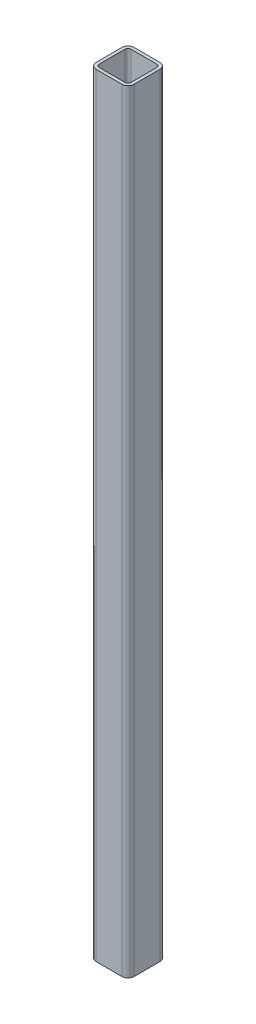
SolidWorks part; units mm, degrees
material "Q235B"
ref_plane "Front Plane" through (0, 0, 0) normal (0, 0, 1) x (1, 0, 0)
ref_plane "Top Plane" through (0, 0, 0) normal (0, 1, 0) x (1, 0, 0)
ref_plane "Right Plane" through (0, 0, 0) normal (1, 0, 0) x (0, 0, -1)
sketch "草图1" plane through (0, 0, 0) normal (0, 0, 1) x (1, 0, 0)
  line L0 (0, 0) -> (0, 1020)
  dimension "D1" = 1020
other "Gb／t 6728—2002 square hollow section 50×50×4(1)"
ref_plane "Plane1" through (0, 0, 0) normal (0, 1, 0) x (-1, 0, 0)
sketch "Sketch1" plane through (0, 0, 0) normal (0, 1, 0) x (-1, 0, 0)
  line L0 (-17, -21) -> (17, -21)
  line L1 (-21, -17) -> (-21, 17)
  line L2 (17, 21) -> (-17, 21)
  line L3 (21, 17) -> (21, -17)
  line L4 (-17, -25) -> (17, -25)
  line L5 (-25, -17) -> (-25, 17)
  line L6 (17, 25) -> (-17, 25)
  line L7 (25, 17) -> (25, -17)
  arc A0 (25, 17) -> (17, 25) centre (17, 17) ccw
  arc A1 (17, -25) -> (25, -17) centre (17, -17) ccw
  arc A2 (-25, -17) -> (-17, -25) centre (-17, -17) ccw
  arc A3 (-17, 25) -> (-25, 17) centre (-17, 17) ccw
  arc A4 (-17, 21) -> (-21, 17) centre (-17, 17) ccw
  arc A5 (21, 17) -> (17, 21) centre (17, 17) ccw
  arc A6 (17, -21) -> (21, -17) centre (17, -17) ccw
  arc A7 (-21, -17) -> (-17, -21) centre (-17, -17) ccw
  point P0 (-25, 0)
  point P1 (25, 0)
  point P2 (0, 25)
  point P3 (0, -25)
  point P4 (0, 0)
  point P5 (-25, -25)
  point P6 (25, -25)
  point P7 (25, 25)
  point P8 (-25, 25)
  point P33 (0, 0)
  dimension "D1" = 8
  dimension "Thickness" = 4
  dimension "V_leg" = 50
